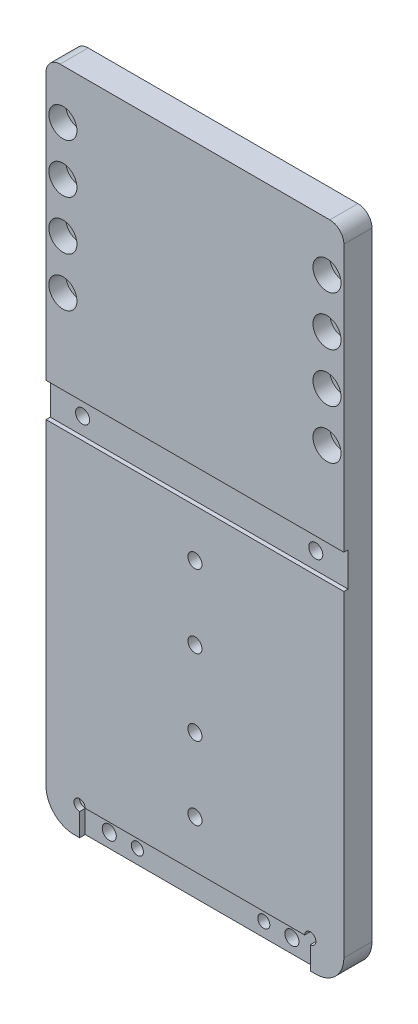
SolidWorks part; units mm, degrees
material "6061铝"
ref_plane "前视基准面" through (0, 0, 0) normal (0, 0, 1) x (1, 0, 0)
ref_plane "上视基准面" through (0, 0, 0) normal (0, 1, 0) x (1, 0, 0)
ref_plane "右视基准面" through (0, 0, 0) normal (1, 0, 0) x (0, 0, -1)
sketch "草图1" plane through (0, 0, 0) normal (0, 0, 1) x (1, 0, 0)
  line L0 (-40, 0) -> (40, 0)
  line L1 (-40, 0) -> (-40, -235)
  line L4 (-40, -235) -> (40, -235)
  line L7 (40, -235) -> (40, 0)
  dimension "D1" = 80
  dimension "D4" = 235
extrude "凸台-拉伸1" add sketch "草图1" along normal blind 10
sketch "草图20" plane through (0, 0, 10) normal (0, 0, 1) x (1, 0, 0)
  line L0 (-40, -235) -> (40, -235) construction
  line L1 (41, -239.1193) -> (-41, -239.1193)
  line L2 (41, -239.1193) -> (41, -224.9)
  line L3 (41, -224.9) -> (-41, -224.9)
  line L4 (-41, -239.1193) -> (-41, -224.9)
  line L5 (41, -239.1193) -> (-41, -224.9) construction
  line L6 (41, -224.9) -> (-41, -239.1193) construction
  point P0 (0, -232.0096)
  dimension "D1" = 10.1
  dimension "D2" = 82
extrude "切除-拉伸3" cut sketch "草图20" against normal blind 2
hole_wizard "打孔尺寸(%根据)开槽圆柱头螺钉的类型4" positions "草图23" profile "草图22" counterbore size "M4" standard "GB" end condition through all
sketch "草图23" plane through (0, 0, 0) normal (0, 0, -1) x (-1, 0, 0)
  line L0 (-22.5, -230) -> (22.5, -230) construction
  line L3 (0, -230) -> (0, 0) construction
  line L6 (40, -235) -> (-40, -235) construction
  point P0 (-22.5, -230)
  point P2 (22.5, -230)
  dimension "D1" = 45
  dimension "D2" = 5
sketch "草图22" plane through (22.5, -230, 0) normal (1, 0, 0) x (0, 1, 0)
  line L0 (0, 0) -> (0, 10)
  line L1 (0, 10) -> (2.15, 10)
  line L3 (2.15, 10) -> (2.15, 5)
  line L4 (2.15, 5) -> (4, 5)
  line L5 (4, 5) -> (4, 0)
  line L7 (4, 0) -> (0, 0)
  line L11 (0, -6.35) -> (0, 107.95) construction
  dimension "通孔孔直径" = 4.3
  dimension "通孔孔深度" = 10
  dimension "柱形沉头孔直径" = 8
  dimension "柱形沉头孔深度" = 5
sketch "草图26" plane through (0, 0, 10) normal (0, 0, 1) x (1, 0, 0)
  line L1 (40, 0) -> (53, 0)
  line L2 (40, 0) -> (40, -87.5)
  line L3 (40, -87.5) -> (53, -87.5)
  line L4 (53, 0) -> (53, -87.5)
  dimension "D1" = 87.5
  dimension "D2" = 53
extrude "凸台-拉伸3" add sketch "草图26" against normal up to surface (10 mm away) up to face at (18.5, -230, 0)
mirror "镜向1" about plane through (0, 0, 0) normal (1, 0, 0) of "凸台-拉伸3"
fillet "圆角5" radius 5 2 edges at (-53, 0, 5) (53, 0, 5)
hole_wizard "打孔尺寸(%根据)内六角圆柱头螺钉的类型1" positions "草图27" profile "草图28" counterbore size "M5" standard "GB" end condition through all
sketch "草图27" plane through (0, 0, 10) normal (0, 0, 1) x (1, 0, 0)
  line L0 (0, 0) -> (0, -60.4975) construction
  line L6 (48, 0) -> (-48, 0) construction
  point P0 (-47, -17.5)
  point P2 (-47, -52.5)
  point P4 (47, -52.5)
  point P6 (47, -17.5)
  dimension "D1" = 94
  dimension "D2" = 35
  dimension "D3" = 17.5
sketch "草图28" plane through (-47, -17.5, 10) normal (1, 0, 0) x (0, -1, 0)
  line L0 (0, 0) -> (0, 10)
  line L1 (0, 10) -> (2.7, 10)
  line L3 (2.7, 10) -> (2.7, 6)
  line L4 (2.7, 6) -> (5, 6)
  line L5 (5, 6) -> (5, 0)
  line L7 (5, 0) -> (0, 0)
  line L11 (0, -6.35) -> (0, 107.95) construction
  dimension "通孔孔直径" = 5.4
  dimension "通孔孔深度" = 10
  dimension "柱形沉头孔直径" = 10
  dimension "柱形沉头孔深度" = 6
pattern_linear "阵列(线性)2" count 2 spacing 17.5 along (0, -1, 0) of "打孔尺寸(%根据)内六角圆柱头螺钉的类型1"
other "移动面1" face at (40, -182.4667, 6) face at (-40, -182.4667, 6) parameters "D1"=13
sketch "草图30" plane through (0, 0, 10) normal (0, 0, 1) x (1, 0, 0)
  line L0 (48, 0) -> (-48, 0) construction
  line L1 (-201.2569, -99.95) -> (64.1287, -99.95)
  line L2 (-201.2569, -99.95) -> (-201.2569, -112.05)
  line L3 (-201.2569, -112.05) -> (64.1287, -112.05)
  line L4 (64.1287, -99.95) -> (64.1287, -112.05)
  line L5 (-201.2569, -99.95) -> (64.1287, -112.05) construction
  line L6 (-201.2569, -112.05) -> (64.1287, -99.95) construction
  point P0 (-68.5641, -106)
  dimension "D1" = 106
  dimension "D2" = 12.1
extrude "切除-拉伸7" cut sketch "草图30" against normal blind 1.5
sketch "草图31" plane through (0, 0, 10) normal (0, 0, 1) x (1, 0, 0)
  line L0 (0, 0) -> (0, -372.2641) construction
  line L1 (-53, -235) -> (-41.05, -235)
  line L2 (-53, -235) -> (-53, -217.4603)
  line L3 (-53, -217.4603) -> (-41.05, -217.4603)
  line L4 (-41.05, -235) -> (-41.05, -217.4603)
  line L5 (53, -235) -> (41.05, -235)
  line L6 (53, -235) -> (53, -214.2151)
  line L7 (53, -214.2151) -> (41.05, -214.2151)
  line L8 (41.05, -235) -> (41.05, -214.2151)
  dimension "D1" = 82.1
extrude "凸台-拉伸4" add sketch "草图31" against normal up to surface (10 mm away) up to face at (-44.3, -70, 0)
sketch "草图32" plane through (0, 0, 10) normal (0, 0, 1) x (1, 0, 0)
  line L0 (41.05, -224.9) -> (-41.05, -224.9) construction
  line L1 (41.05, -224.9) -> (-41.05, -224.9) construction
  circle A0 centre (-41.05, -224.9) radius 2
  circle A1 centre (41.05, -224.9) radius 2
  dimension "D1" = 4
extrude "切除-拉伸8" cut sketch "草图32" against normal up to surface (2 mm away) up to face at (0, -229.95, 8)
hole_wizard "大小mm 暗销孔1" positions "草图33" profile "草图34" hole size "Ø5.0" standard "GB"
sketch "草图33" plane through (0, 0, 0) normal (0, 0, -1) x (-1, 0, 0)
  point P0 (-32.5, -230)
  point P3 (32.5, -230)
sketch "草图34" plane through (32.5, -230, 0) normal (1, 0, 0) x (0, 1, 0)
  line L0 (0, 0) -> (0, 11.6022)
  line L1 (0, 11.6022) -> (2.5, 10.1)
  line L2 (2.5, 10.1) -> (2.5, 0)
  line L5 (2.5, 0) -> (0, 0)
  line L10 (0, 11.6022) -> (-2.5, 10.1) construction
  line L11 (0, -6.35) -> (0, 107.95) construction
  dimension "孔直径" = 5
  dimension "孔深度" = 10.1
  dimension "导头角度" = 118
fillet "圆角6" radius 10 2 edges at (53, -235, 5) (-53, -235, 5)
hole_wizard "M6 螺纹孔1" positions "草图35" profile "草图37" tap size "M6" standard "GB"
sketch "草图35" plane through (0, 0, 10) normal (0, 0, 1) x (1, 0, 0)
  point P0 (-41.5, -106)
  point P3 (41.5, -106)
sketch "草图37" plane through (-41.5, -106, 10) normal (1, 0, 0) x (0, -1, 0)
  line L0 (0, 0) -> (0, 16.5022)
  line L1 (0, 16.5022) -> (2.5, 15)
  line L2 (2.5, 15) -> (2.5, 0)
  line L5 (2.5, 0) -> (0, 0)
  line L10 (0, 16.5022) -> (-2.5, 15) construction
  line L11 (0, -6.35) -> (0, 107.95) construction
  dimension "螺纹孔钻头直径" = 5
  dimension "螺纹孔钻头深度" = 15
  dimension "导头角度" = 118
cosmetic thread "孔螺蚊线11" parameters "D1"=10, "D2"=6
cosmetic thread "孔螺蚊线12" parameters "D1"=10, "D2"=6
hole_wizard "M6 螺纹孔2" positions "草图38" profile "草图39" tap size "M6" standard "GB"
sketch "草图38" plane through (0, 0, 10) normal (0, 0, 1) x (1, 0, 0)
  line L0 (-41.05, -235) -> (41.05, -235) construction
  line L1 (53, -225) -> (53, -112.05) construction
  point P0 (0, -208)
  dimension "D1" = 27
  dimension "D2" = 53
sketch "草图39" plane through (0, -208, 10) normal (1, 0, 0) x (0, -1, 0)
  line L0 (0, 0) -> (0, 16.5022)
  line L1 (0, 16.5022) -> (2.5, 15)
  line L2 (2.5, 15) -> (2.5, 0)
  line L5 (2.5, 0) -> (0, 0)
  line L10 (0, 16.5022) -> (-2.5, 15) construction
  line L11 (0, -6.35) -> (0, 107.95) construction
  dimension "螺纹孔钻头直径" = 5
  dimension "螺纹孔钻头深度" = 15
  dimension "导头角度" = 118
cosmetic thread "孔螺蚊线13" parameters "D1"=10, "D2"=6
hole_wizard "M6 螺纹孔3" positions "草图40" profile "草图41" tap size "M6" standard "GB" end condition through all
sketch "草图40" plane through (0, 0, 10) normal (0, 0, 1) x (1, 0, 0)
  point P0 (0, -155)
  point P3 (0, -182)
sketch "草图41" plane through (0, -155, 10) normal (1, 0, 0) x (0, -1, 0)
  line L0 (0, 0) -> (0, 10)
  line L1 (0, 10) -> (2.5, 10)
  line L2 (2.5, 10) -> (2.5, 0)
  line L5 (2.5, 0) -> (0, 0)
  line L11 (0, -6.35) -> (0, 107.95) construction
  dimension "通孔螺纹孔钻头直径" = 5
  dimension "通孔螺纹孔钻头深度" = 10
cosmetic thread "孔螺蚊线14" parameters "D2"=6
cosmetic thread "孔螺蚊线15" parameters "D2"=6
hole_wizard "M6 螺纹孔4" positions "草图42" profile "草图43" tap size "M6" standard "GB" end condition through all
sketch "草图42" plane through (0, 0, 10) normal (0, 0, 1) x (1, 0, 0)
  line L0 (0, -127.5) -> (0, -130.5) construction
  point P7 (0, -129)
sketch "草图43" plane through (0, -129, 10) normal (1, 0, 0) x (0, -1, 0)
  line L0 (0, 0) -> (0, 10)
  line L1 (0, 10) -> (2.5, 10)
  line L2 (2.5, 10) -> (2.5, 0)
  line L5 (2.5, 0) -> (0, 0)
  line L11 (0, -6.35) -> (0, 107.95) construction
  dimension "通孔螺纹孔钻头直径" = 5
  dimension "通孔螺纹孔钻头深度" = 10
cosmetic thread "孔螺蚊线16" parameters "D2"=6
